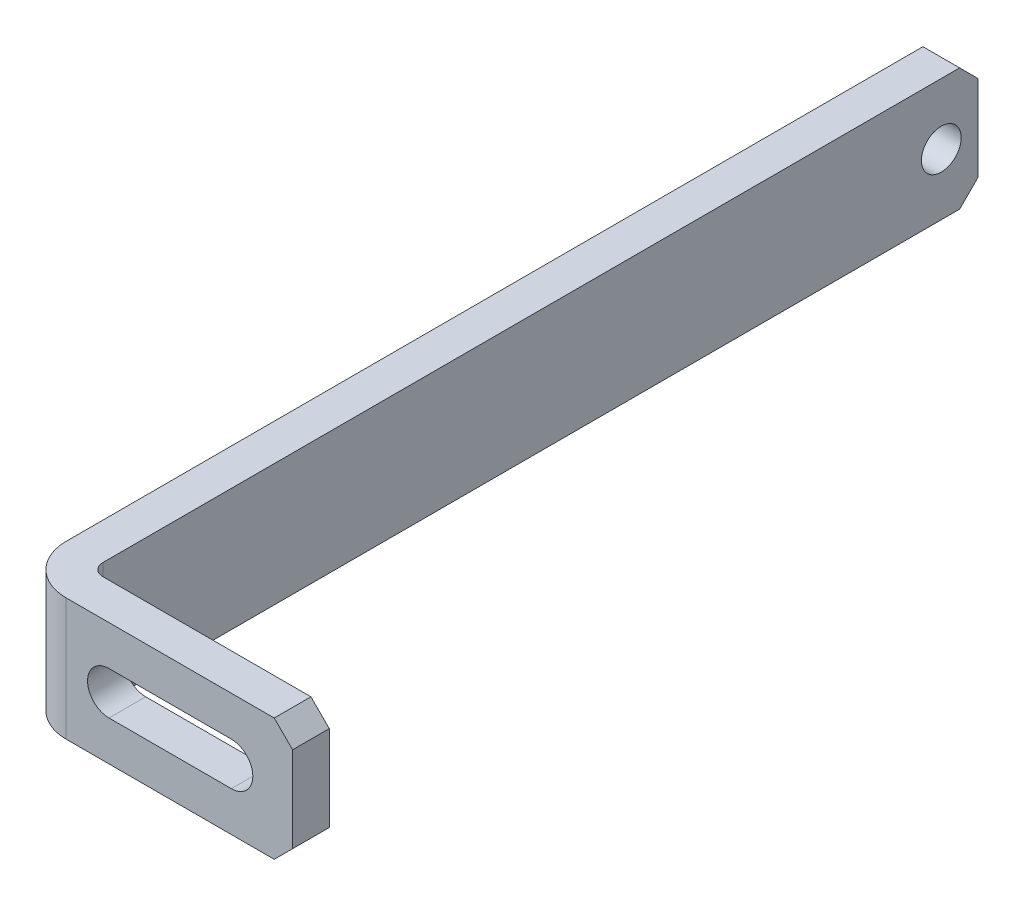
from build123d import *

# Parameters (mm, degrees)
SKETCH1_W           = 45
SKETCH1_H           = 151
BOSS_EXTRUDE1_DEPTH = 20
SKETCH2_W           = 39
SKETCH2_H           = 145
CUT_EXTRUDE1_DEPTH  = 82.280378936
SKETCH3_R           = 3.25
CUT_EXTRUDE2_DEPTH  = 88.299770905
CUT_EXTRUDE3_DEPTH  = 149.092032196
CHAMFER1_SIZE       = 3
FILLET1_R           = 2
FILLET2_R           = 8


with BuildPart() as part:
    # Sketch1 → Boss-Extrude1 (new body)
    with BuildSketch(Plane(origin=(0, 0, 0), x_dir=(1, 0, 0), z_dir=(0, 1, 0))):
        Rectangle(SKETCH1_W, SKETCH1_H)
    extrude(amount=BOSS_EXTRUDE1_DEPTH)

    # Sketch2 → Cut-Extrude1 (cut, through all)
    with BuildSketch(Plane(origin=(0, 20, 0), x_dir=(1, 0, 0), z_dir=(0, 1, 0))):
        with Locations((3, 3)):
            Rectangle(SKETCH2_W, SKETCH2_H)
    extrude(amount=-CUT_EXTRUDE1_DEPTH, mode=Mode.SUBTRACT)

    # Sketch3 → Cut-Extrude2 (cut, through all)
    with BuildSketch(Plane(origin=(-16.5, 0, 0), x_dir=(0, 0, -1), z_dir=(1, 0, 0))):
        with Locations((69.5, 10)):
            Circle(SKETCH3_R)
    extrude(amount=-CUT_EXTRUDE2_DEPTH, mode=Mode.SUBTRACT)

    # Sketch4 → Cut-Extrude3 (cut, through all)
    with BuildSketch(Plane(origin=(0, 0, 69.5), x_dir=(-1, 0, 0), z_dir=(0, 0, -1))):
        with BuildLine():
            Line((-12.5, 13.5), (7.5, 13.5))
            ThreePointArc((7.5, 13.5), (11, 10), (7.5, 6.5))
            Line((7.5, 6.5), (-12.5, 6.5))
            ThreePointArc((-12.5, 6.5), (-16, 10), (-12.5, 13.5))
        make_face()
    extrude(amount=-CUT_EXTRUDE3_DEPTH, mode=Mode.SUBTRACT)

    # Chamfer1
    chamfer1_edges = [part.edges().sort_by_distance(p)[0] for p in [
        (22.5, 20, 72.5),
        (-19.5, 0, -75.5),
        (-19.5, 20, -75.5),
        (22.5, 0, 72.5),
    ]]
    chamfer(chamfer1_edges, length=CHAMFER1_SIZE)

    # Fillet1
    fillet1_edges = [part.edges().sort_by_distance(p)[0] for p in [
        (-16.5, 10, 69.5),
    ]]
    fillet(fillet1_edges, radius=FILLET1_R)

    # Fillet2
    fillet2_edges = [part.edges().sort_by_distance(p)[0] for p in [
        (-22.5, 10, 75.5),
    ]]
    fillet(fillet2_edges, radius=FILLET2_R)


solid = part.part
